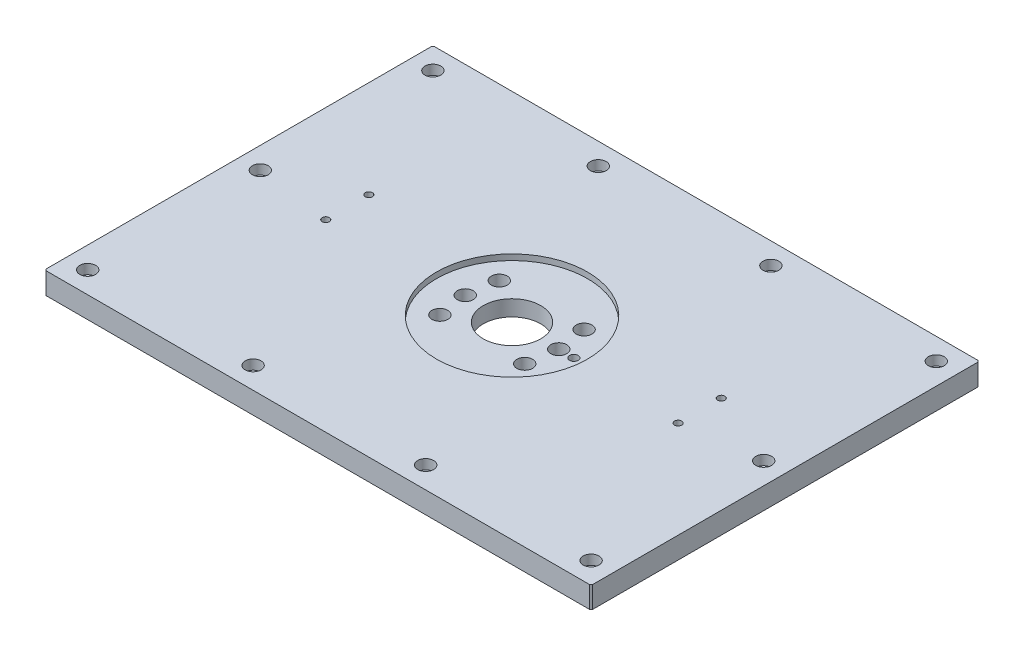
from build123d import *

# Parameters (mm, degrees)
SKETCH_1_W                = 380
SKETCH_1_H                = 270
EXTRUDE_1_DEPTH           = 7.5
CHAMFER_1_SIZE            = 1
SKETCH_2_R                = 20
CUT_EXTRUDE_1_DEPTH       = 15
HOLE_WIZARD_3_D           = 6.6
HOLE_WIZARD_3_CBORE_D     = 11
HOLE_WIZARD_3_CBORE_DEPTH = 6.8
SKETCH_9_R                = 5.5
CUT_EXTRUDE_2_DEPTH       = 234.559414283
SKETCH_11_R               = 52.5
CUT_EXTRUDE_3_DEPTH       = 4
HOLE_WIZARD_M6_1_D        = 5
SKETCH_15_R               = 3
CUT_EXTRUDE_4_DEPTH       = 9


with BuildPart() as part:
    # 草图1 → 凸台-拉伸1 (new, symmetric)
    with BuildSketch(Plane(origin=(0, 0, 0), x_dir=(1, 0, 0), z_dir=(0, 1, 0))):
        Rectangle(SKETCH_1_W, SKETCH_1_H)
    extrude(amount=EXTRUDE_1_DEPTH, both=True)

    # 倒角1
    chamfer_1_edges = [part.edges().sort_by_distance(p)[0] for p in [
        (190, 0, 135),
        (-190, 0, 135),
        (-190, 0, -135),
        (190, 0, -135),
    ]]
    chamfer(chamfer_1_edges, length=CHAMFER_1_SIZE)

    # 草图2 → 切除-拉伸1 (cut)
    with BuildSketch(Plane(origin=(0, 7.5, 0), x_dir=(1, 0, 0), z_dir=(0, 1, 0))):
        with Locations(Location((0, 0, 0), (0, 0, 270))):
            Circle(SKETCH_2_R)
    extrude(amount=-CUT_EXTRUDE_1_DEPTH, mode=Mode.SUBTRACT)

    # 打孔尺寸(%根据)内六角圆柱头螺钉的类型3 (through all)
    with Locations(Plane(origin=(0, 7.5, 0), x_dir=(1, 0, 0), z_dir=(0, 1, 0))):
        with Locations((-175, 120), (-60, 120), (-60, -120), (-175, 0), (-175, -120), (175, -120), (175, 0), (60, -120), (60, 120), (175, 120)):
            CounterBoreHole(HOLE_WIZARD_3_D / 2, HOLE_WIZARD_3_CBORE_D / 2, HOLE_WIZARD_3_CBORE_DEPTH)

    # 草图9 → 切除-拉伸2 (cut, through all)
    with BuildSketch(Plane(origin=(0, 7.5, 0), x_dir=(1, 0, 0), z_dir=(0, 1, 0))):
        with Locations(Location((-29.489473594, 20.648751709, 0), (0, 0, 270))):
            Circle(SKETCH_9_R)
        with Locations(Location((-29.489473594, -20.648751709, 0), (0, 0, 270))):
            Circle(SKETCH_9_R)
        with Locations(Location((-32.5, 0, 0), (0, 0, 270))):
            Circle(SKETCH_9_R)
        with Locations(Location((29.489473594, -20.648751709, 0), (0, 0, 90))):
            Circle(SKETCH_9_R)
        with Locations(Location((32.5, 0, 0), (0, 0, 90))):
            Circle(SKETCH_9_R)
        with Locations(Location((29.489473594, 20.648751709, 0), (0, 0, 90))):
            Circle(SKETCH_9_R)
    extrude(amount=-CUT_EXTRUDE_2_DEPTH, mode=Mode.SUBTRACT)

    # 草图11 → 切除-拉伸3 (cut)
    with BuildSketch(Plane(origin=(0, 7.5, 0), x_dir=(1, 0, 0), z_dir=(0, 1, 0))):
        with Locations(Location((0, 0, 0), (0, 0, 270))):
            Circle(SKETCH_11_R)
    extrude(amount=-CUT_EXTRUDE_3_DEPTH, mode=Mode.SUBTRACT)

    # M6 螺纹孔1 (through all)
    with Locations(Plane(origin=(0, 7.5, 0), x_dir=(1, 0, 0), z_dir=(0, 1, 0))):
        with Locations((122.5, -7), (122.5, 23), (-122.5, 23), (-122.5, -7)):
            Hole(HOLE_WIZARD_M6_1_D / 2)

    # 草图15 → 切除-拉伸4 (cut)
    with BuildSketch(Plane(origin=(0, 3.5, 0), x_dir=(1, 0, 0), z_dir=(0, 1, 0))):
        with Locations(Location((43, 0, 0), (0, 0, 270))):
            Circle(SKETCH_15_R)
    extrude(amount=-CUT_EXTRUDE_4_DEPTH, mode=Mode.SUBTRACT)


solid = part.part
